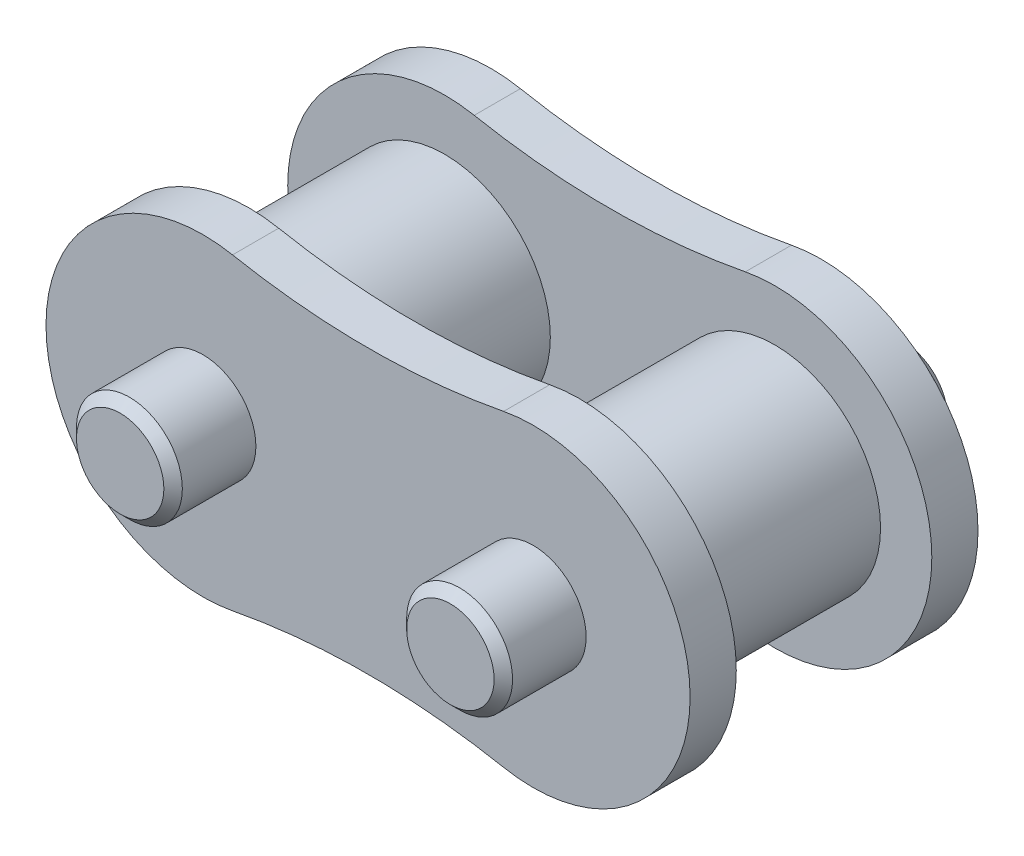
SolidWorks part; units mm, degrees
ref_plane "前视基准面" through (0, 0, 0) normal (0, 0, 1) x (1, 0, 0)
ref_plane "上视基准面" through (0, 0, 0) normal (0, 1, 0) x (1, 0, 0)
ref_plane "右视基准面" through (0, 0, 0) normal (1, 0, 0) x (0, 0, -1)
sketch "草图1" plane through (0, 0, 0) normal (0, 0, 1) x (1, 0, 0)
  line L0 (-7.9375, 0) -> (7.9375, 0) construction
  line L1 (0, 6.7905) -> (0, -6.7905) construction
  line L2 (7.9375, 0) -> (21.7775, 0) construction
  line L3 (21.7775, 0) -> (31.1775, 0) construction
  circle A0 centre (-7.9375, 0) radius 7.545
  circle A1 centre (7.9375, 0) radius 7.545
  circle A2 centre (0, 41.3748) radius 34.5843
  circle A3 centre (0, -41.3748) radius 34.5843
  circle A4 centre (-7.9375, 0) radius 5.08
  circle A5 centre (7.9375, 0) radius 5.08
  circle A6 centre (-7.9375, 0) radius 2.545
  circle A7 centre (7.9375, 0) radius 2.545
  point P16 (29.7375, 0)
  point P18 (26.0475, 0)
  point P19 (9.9375, 0)
sketch "草图2" plane through (0, 0, 0) normal (0, 0, 1) x (1, 0, 0)
  circle A0 centre (7.9375, 0) radius 5.08 construction
  circle A1 centre (-7.9375, 0) radius 5.08 construction
  circle A2 centre (7.9375, 0) radius 5.08
  circle A3 centre (-7.9375, 0) radius 5.08
extrude "拉伸1" add sketch "草图2" along normal mid plane 9.4
sketch "草图3" plane through (0, 0, 4.7) normal (0, 0, 1) x (1, 0, 0)
  circle A0 centre (-7.9375, 0) radius 7.545 construction
  arc A1 (-6.516, 7.4099) -> (-6.516, -7.4099) centre (-7.9375, 0) ccw
  circle A2 centre (7.9375, 0) radius 7.545 construction
  arc A3 (6.516, -7.4099) -> (6.516, 7.4099) centre (7.9375, 0) ccw
  circle A4 centre (0, 41.3748) radius 34.5843 construction
  arc A5 (-6.516, 7.4099) -> (6.516, 7.4099) centre (0, 41.3748) ccw
  circle A6 centre (0, -41.3748) radius 34.5843 construction
  arc A7 (6.516, -7.4099) -> (-6.516, -7.4099) centre (0, -41.3748) ccw
extrude "拉伸2" add sketch "草图3" along normal blind 2.22
mirror "镜向1" about plane through (0, 0, 0) normal (0, 0, 1) of "拉伸2"
sketch "草图5" plane through (0, 0, 0) normal (0, 0, 1) x (1, 0, 0)
  line L0 (7.9375, 0) -> (23.6177, -2.4794) construction
  line L1 (-7.9375, 0) -> (7.9375, 0) construction
  line L2 (-7.9375, 0) -> (-775.7974, -60.3344)
  line L4 (0, -101.0185) -> (-770.3833, -129.2378) construction
  line L5 (23.6177, -2.4794) -> (38.7182, -7.3775) construction
  arc A0 (26.3679, -198.8575) -> (-7.9375, 0) centre (0, -101.0185) ccw
  arc A1 (-775.7974, -60.3344) -> (-788.8625, -195.8375) centre (-770.3833, -129.2378) ccw
  arc A2 (-788.8625, -195.8375) -> (26.3679, -198.8575) centre (-375.7258, 1293.1233) ccw
  dimension "R2" = 202.6597
  dimension "R1" = 138.2317
  dimension "a" = 770.9
  dimension "La" = 770.2266
  dimension "L2" = 299.6078
  dimension "L" = 825
  dimension "L1" = 193.0074
curve "组合曲线1"
sketch "草图4" plane through (0, 0, 0) normal (0, 0, 1) x (1, 0, 0)
  circle A0 centre (7.9375, 0) radius 2.545 construction
  circle A1 centre (-7.9375, 0) radius 2.545 construction
  circle A2 centre (7.9375, 0) radius 2.545
  circle A3 centre (-7.9375, 0) radius 2.545
extrude "拉伸3" add sketch "草图4" against normal mid plane 21.8
chamfer "倒角1" distance 0.444 angle 45 4 edges at (10.4825, 0, -10.9) (-5.3925, 0, -10.9) (10.4825, 0, 10.9) (-5.3925, 0, 10.9)
equation "\"D1@拉伸1\" = \"b1@草图1\""
equation "\"D1@拉伸2\" = (  \"b2@草图1\" - \"D1@拉伸1\" )  / 2"
equation "\"D1@拉伸3\" = \"b4@草图1\""
equation "\"D1@倒角1\" = \"D1@拉伸2\" / 5"
equation "\"h3@草图1\" = \"h2@草图1\" * 0.9"
